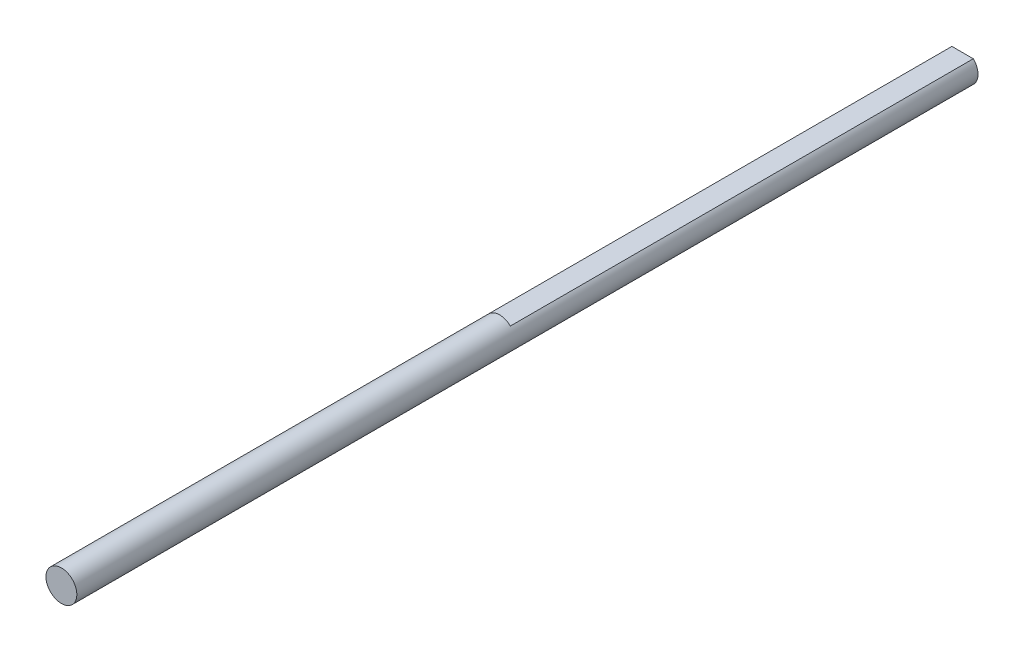
SolidWorks part; units mm, degrees
ref_plane "Front Plane" through (0, 0, 0) normal (0, 0, 1) x (1, 0, 0)
ref_plane "Top Plane" through (0, 0, 0) normal (0, 1, 0) x (1, 0, 0)
ref_plane "Right Plane" through (0, 0, 0) normal (1, 0, 0) x (0, 0, -1)
other "Configuration Table"
sketch "Sketch1" plane through (0, 0, 0) normal (0, 0, 1) x (1, 0, 0)
  circle A0 centre (0, 0) radius 2.5
extrude "Boss-Extrude1" add sketch "Sketch1" along normal blind 162
sketch "Sketch2" plane through (0, 0, 0) normal (0, 0, -1) x (-1, 0, 0)
  line L0 (0, 0) -> (0, 1.8) construction
  line L1 (0, 1.8) -> (1.7349, 1.8)
  line L2 (0, 1.8) -> (-1.7349, 1.8)
  circle A1 centre (0, 0) radius 2.5 construction
  arc A2 (1.7349, 1.8) -> (-1.7349, 1.8) centre (0, 0) ccw
  dimension "D1" = 1.8
extrude "Cut-Extrude1" cut sketch "Sketch2" against normal blind 75
sketch "Sketch3" plane through (0, 0, 162) normal (0, 0, 1) x (1, 0, 0)
  circle A1 centre (0, 0) radius 2.5
  circle A2 centre (0, 0) radius 2.5
  dimension "D1" = 0
extrude "Cut-Extrude2" cut sketch "Sketch3" against normal blind 16
